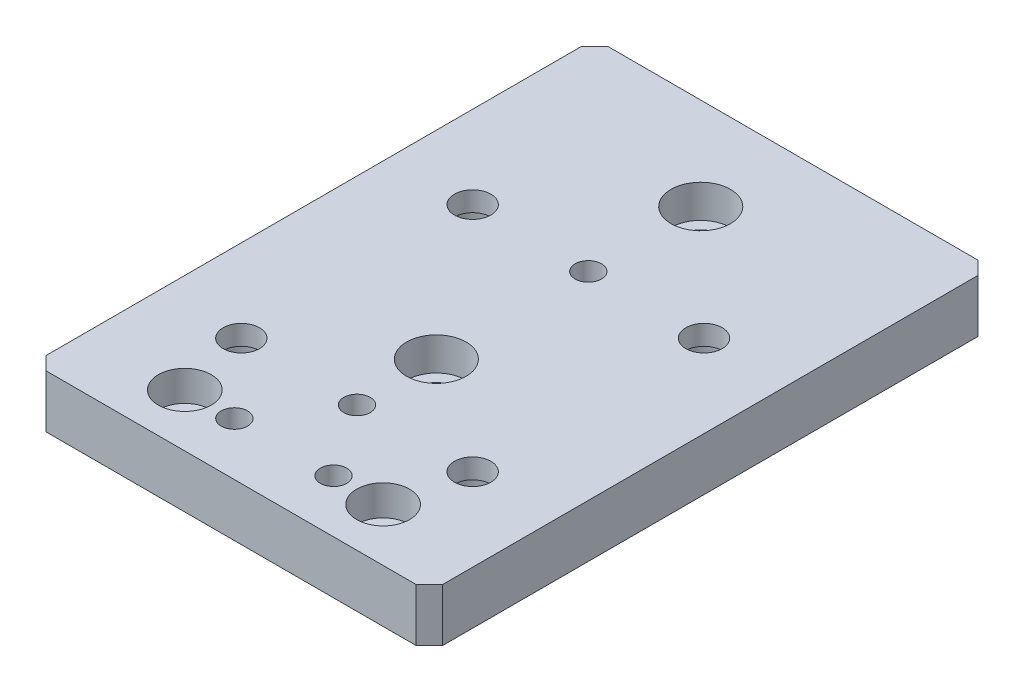
from build123d import *

# Parameters (mm, degrees)
SKETCH_1_W                  = 60
SKETCH_1_H                  = 85
EXTRUDE_1_DEPTH             = 8
HOLE_WIZARD_1_D             = 5.5
HOLE_WIZARD_1_CBORE_D       = 9
HOLE_WIZARD_1_CBORE_DEPTH   = 5
HOLE_WIZARD_2_D             = 5.5
HOLE_WIZARD_2_DEPTH         = 12.4
HOLE_WIZARD_2_CBORE_D       = 9
HOLE_WIZARD_2_CBORE_DEPTH   = 5
HOLE_WIZARD_2_TIP           = 1.652366702
HOLE_WIZARD_1_2_D           = 4.5
HOLE_WIZARD_1_2_CBORE_D     = 8
HOLE_WIZARD_1_2_CBORE_DEPTH = 4.6
HOLE_WIZARD_4_0_4_1_D       = 4
CHAMFER_1_SIZE              = 2


with BuildPart() as part:
    # 草图1 → 凸台-拉伸1 (new body)
    with BuildSketch(Plane(origin=(0, 0, 0), x_dir=(1, 0, 0), z_dir=(0, 1, 0))):
        Rectangle(SKETCH_1_W, SKETCH_1_H)
    extrude(amount=EXTRUDE_1_DEPTH)

    # Hole Wizard 1 (through all)
    with Locations(Plane(origin=(0, 0, 0), x_dir=(-1, 0, 0), z_dir=(0, -1, 0))):
        with Locations((17.5, -23.45), (-17.5, -23.45), (17.5, 11.55), (-17.5, 11.55)):
            CounterBoreHole(HOLE_WIZARD_1_D / 2, HOLE_WIZARD_1_CBORE_D / 2, HOLE_WIZARD_1_CBORE_DEPTH)

    # 大小六角凹头盖螺钉柱孔2
    with Locations(Plane(origin=(0, 8, 0), x_dir=(1, 0, 0), z_dir=(0, 1, 0))):
        with Locations((0, 28.554479799), (0, -11.445520201)):
            CounterBoreHole(HOLE_WIZARD_2_D / 2, HOLE_WIZARD_2_CBORE_D / 2, HOLE_WIZARD_2_CBORE_DEPTH, depth=HOLE_WIZARD_2_DEPTH)
            with Locations((0, 0, -(HOLE_WIZARD_2_DEPTH + HOLE_WIZARD_2_TIP / 2))):  # 118° drill point
                Cone(0, HOLE_WIZARD_2_D / 2, HOLE_WIZARD_2_TIP, mode=Mode.SUBTRACT)

    # Hole Wizard 1 2 (through all)
    with Locations(Plane(origin=(0, 8, 0), x_dir=(1, 0, 0), z_dir=(0, 1, 0))):
        with Locations((-15, -34.5), (15, -34.5)):
            CounterBoreHole(HOLE_WIZARD_1_2_D / 2, HOLE_WIZARD_1_2_CBORE_D / 2, HOLE_WIZARD_1_2_CBORE_DEPTH)

    # Ø4.0 (4) 直径孔1 (through all)
    with Locations(Plane(origin=(0, 8, 0), x_dir=(1, 0, 0), z_dir=(0, 1, 0))):
        with Locations((-7.5, -34.5), (7.5, -34.5), (0, -23.45), (0, 11.55)):
            Hole(HOLE_WIZARD_4_0_4_1_D / 2)

    # 倒角1
    chamfer_1_edges = [part.edges().sort_by_distance(p)[0] for p in [
        (30, 4, 42.5),
        (-30, 4, 42.5),
        (-30, 4, -42.5),
        (30, 4, -42.5),
    ]]
    chamfer(chamfer_1_edges, length=CHAMFER_1_SIZE)


solid = part.part
